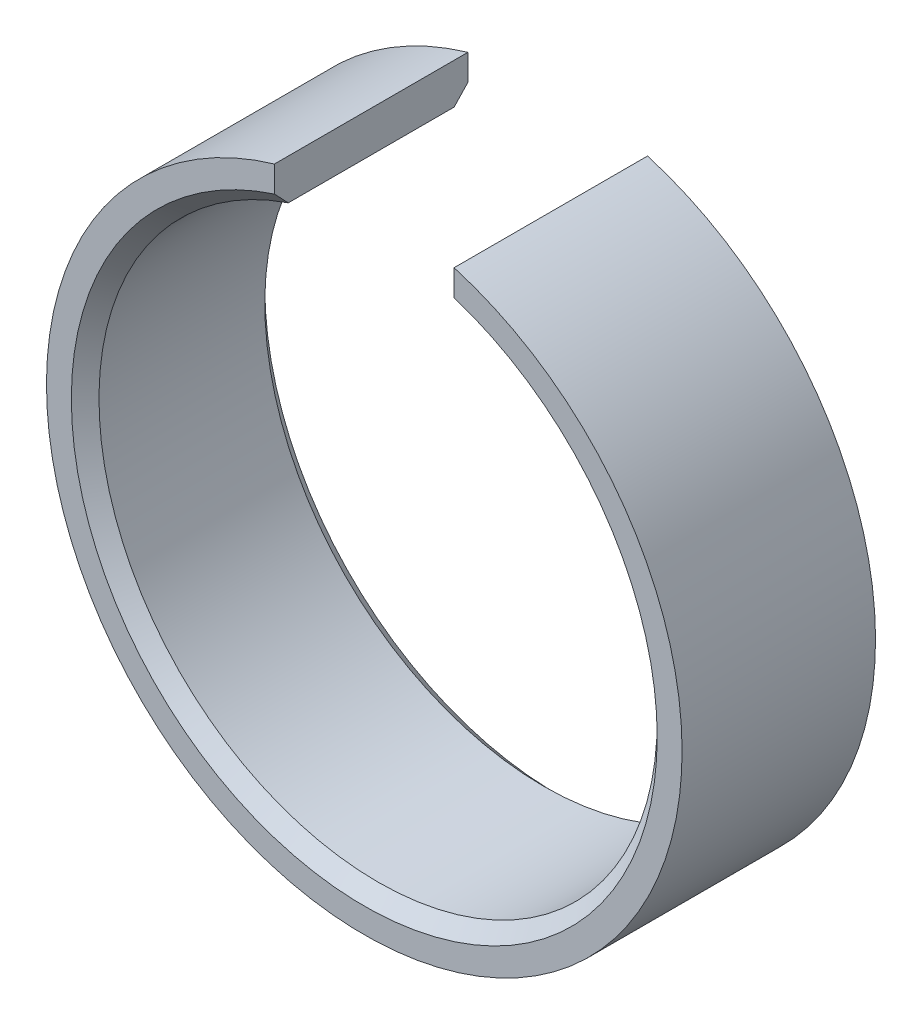
SolidWorks part; units mm, degrees
material "6061-T6 (GB)"
ref_plane "Front Plane" through (0, 0, 0) normal (0, 0, 1) x (1, 0, 0)
ref_plane "Top Plane" through (0, 0, 0) normal (0, 1, 0) x (1, 0, 0)
ref_plane "Right Plane" through (0, 0, 0) normal (1, 0, 0) x (0, 0, -1)
sketch "Sketch1" plane through (0, 0, 0) normal (0, 0, 1) x (1, 0, 0)
  circle A0 centre (0, 0) radius 10.1
  circle A1 centre (0, 0) radius 11.5
  dimension "D1" = 20.2
  dimension "D2" = 23
extrude "Boss-Extrude1" add sketch "Sketch1" along normal blind 7
sketch "Sketch2" plane through (0, 0, 7) normal (0, 0, 1) x (1, 0, 0)
  line L0 (0, 0) -> (0, 10.1) construction
  line L1 (3.25, 0) -> (-3.25, 0)
  line L2 (3.25, 0) -> (3.25, 15)
  line L3 (3.25, 15) -> (-3.25, 15)
  line L4 (-3.25, 0) -> (-3.25, 15)
  line L5 (3.25, 0) -> (-3.25, 15) construction
  line L6 (3.25, 15) -> (-3.25, 0) construction
  circle A0 centre (0, 0) radius 10.1 construction
  point P0 (0, 7.5)
  dimension "D1" = 6.5
  dimension "D2" = 15
extrude "Cut-Extrude1" cut sketch "Sketch2" against normal through all
chamfer "Chamfer1" distance 0.5 angle 45 2 edges at (0, -10.1, 0) (0, -10.1, 7)
